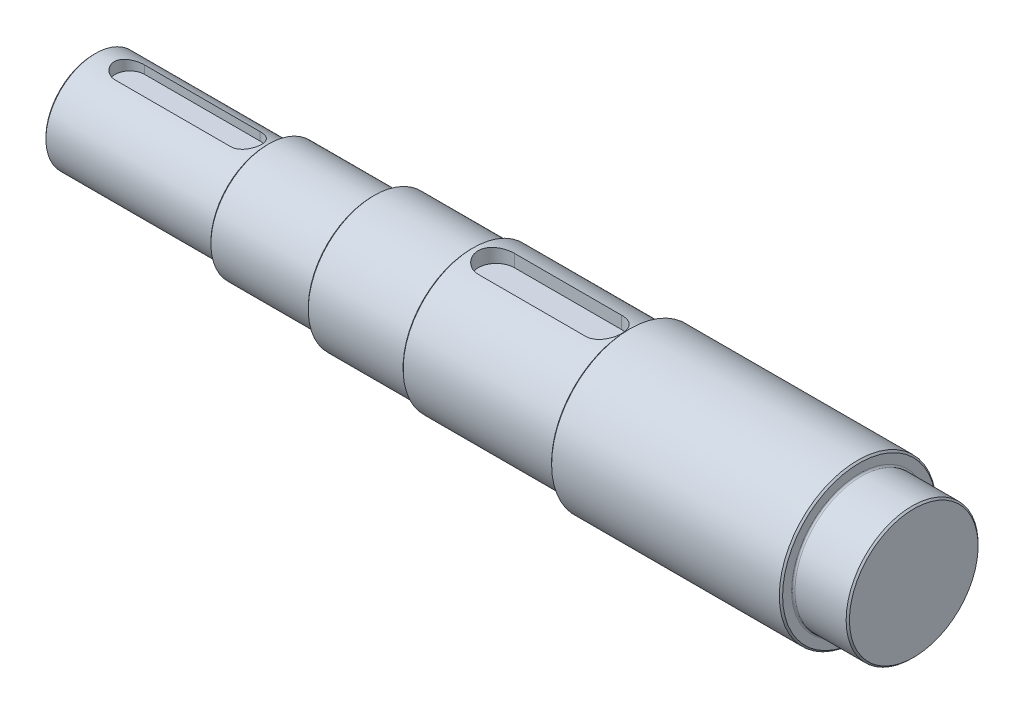
SolidWorks part; units mm, degrees
ref_plane "Front Plane" through (0, 0, 0) normal (0, 0, 1) x (1, 0, 0)
ref_plane "Top Plane" through (0, 0, 0) normal (0, 1, 0) x (1, 0, 0)
ref_plane "Right Plane" through (0, 0, 0) normal (1, 0, 0) x (0, 0, -1)
other "Configuration Table"
sketch "Sketch1" plane through (0, 0, 0) normal (0, 0, 1) x (1, 0, 0)
  line L0 (-10.3235, 0) -> (538.2344, 0) construction
  line L1 (0, 0) -> (0, 30)
  line L2 (0, 30) -> (105, 30)
  line L3 (105, 30) -> (105, 35)
  line L4 (105, 35) -> (169, 35)
  line L5 (169, 35) -> (169, 40)
  line L6 (169, 40) -> (229, 40)
  line L7 (229, 40) -> (229, 42.5)
  line L8 (229, 42.5) -> (324, 42.5)
  line L9 (324, 42.5) -> (324, 47.5)
  line L10 (324, 47.5) -> (464, 47.5)
  line L11 (464, 47.5) -> (464, 40)
  line L12 (464, 40) -> (497, 40)
  line L13 (497, 40) -> (497, 0)
  line L14 (0, 0) -> (497, 0)
  dimension "D1" = 105
  dimension "D2" = 64
  dimension "D3" = 60
  dimension "D4" = 95
  dimension "D5" = 33
  dimension "D6" = 497
  dimension "D7" = 30
  dimension "D8" = 35
  dimension "D9" = 40
  dimension "D10" = 42.5
  dimension "D11" = 47.5
  dimension "D12" = 40
revolve "Revolve2" add sketch "Sketch1" angle 360 about L0
ref_plane "Plane2" through (0, 42.5, 0) normal (0, 1, 0) x (1, 0, 0)
sketch "Sketch2" plane through (0, 42.5, 0) normal (0, 1, 0) x (1, 0, 0)
  line L0 (-24.9412, 0) -> (552.5826, 0) construction
  line L1 (309, 11) -> (244, 11)
  line L2 (244, -11) -> (309, -11)
  line L3 (324, 42.5) -> (324, -42.5) construction
  arc A0 (244, 11) -> (244, -11) centre (244, 0) ccw
  arc A1 (309, -11) -> (309, 11) centre (309, 0) ccw
  point P9 (233, 0)
  dimension "D1" = 76
  dimension "D2" = 22
  dimension "D3" = 15
extrude "Cut-Extrude2" cut sketch "Sketch2" against normal blind 9
ref_plane "Plane4" through (0, 30, 0) normal (0, 1, 0) x (1, 0, 0)
sketch "Sketch4" plane through (0, 30, 0) normal (0, 1, 0) x (1, 0, 0)
  line L0 (90, 10.9054) -> (20, 10.9054)
  line L1 (20, -7.0946) -> (90, -7.0946)
  line L2 (105, 30) -> (105, -30) construction
  arc A0 (20, 10.9054) -> (20, -7.0946) centre (20, 1.9054) ccw
  arc A1 (90, -7.0946) -> (90, 10.9054) centre (90, 1.9054) ccw
  point P6 (99, 1.9054)
  point P7 (11, 1.9054)
  dimension "D1" = 18
  dimension "D2" = 88
  dimension "D3" = 15
extrude "Cut-Extrude3" cut sketch "Sketch4" against normal blind 7
chamfer "Chamfer1" distance 1 angle 45 7 edges at (497, 0, 40) (464, 0, 47.5) (324, 0, 47.5) (229, 0, 42.5) (169, 0, 40) (105, 0, 35) (0, 0, 30)
fillet "Fillet1" radius 1 5 edges at (105, 0, 30) (169, 0, 35) (229, 0, 40) (324, 0, 42.5) (464, 0, 40)
